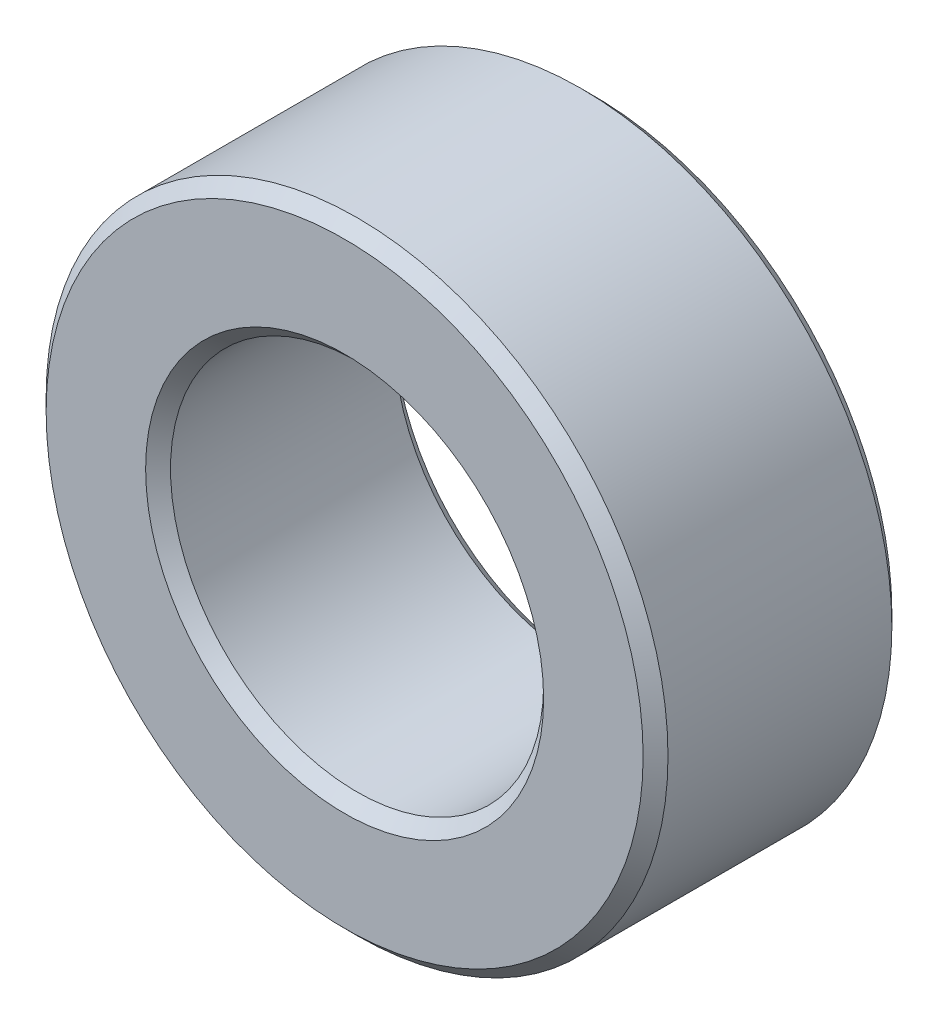
from build123d import *

# Parameters (mm, degrees)
SKETCH1_R           = 25
SKETCH1_R_2         = 15
BOSS_EXTRUDE1_DEPTH = 20
CHAMFER1_SIZE       = 1


with BuildPart() as part:
    # Sketch1 → Boss-Extrude1 (new body)
    with BuildSketch(Plane.XY):
        Circle(SKETCH1_R)
        Circle(SKETCH1_R_2, mode=Mode.SUBTRACT)
    extrude(amount=BOSS_EXTRUDE1_DEPTH)

    # Chamfer1
    chamfer1_edges = [part.edges().sort_by_distance(p)[0] for p in [
        (-25, 0, 0),
        (-25, 0, 20),
        (-15, 0, 0),
        (-15, 0, 20),
    ]]
    chamfer(chamfer1_edges, length=CHAMFER1_SIZE)


solid = part.part
